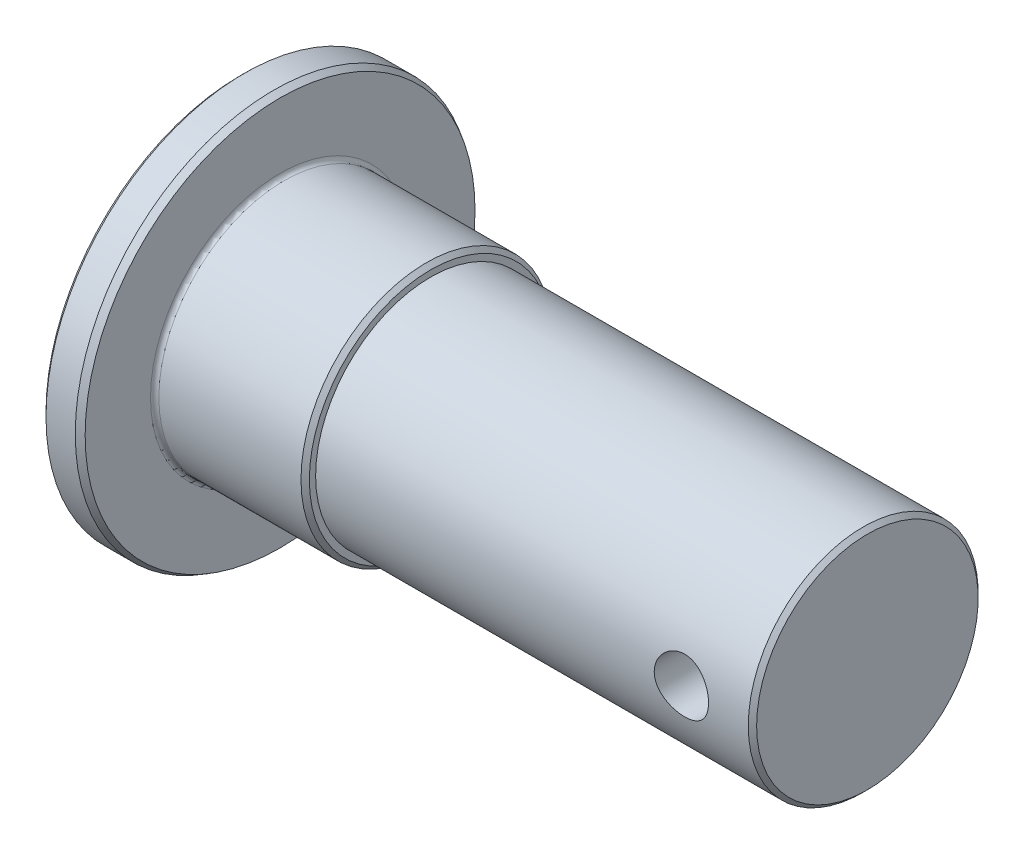
SolidWorks part; units mm, degrees
material "普通碳钢"
ref_plane "Front Plane" through (0, 0, 0) normal (0, 0, 1) x (1, 0, 0)
ref_plane "Top Plane" through (0, 0, 0) normal (0, 1, 0) x (1, 0, 0)
ref_plane "Right Plane" through (0, 0, 0) normal (1, 0, 0) x (0, 0, -1)
sketch "Sketch1" plane through (0, 0, 0) normal (0, 0, 1) x (1, 0, 0)
  line L0 (0, 0) -> (148.8633, 0) construction
  line L1 (0, 0) -> (0, 47.5)
  line L2 (0, -52.25) -> (0, 52.25) construction
  line L3 (0, 47.5) -> (8, 47.5)
  line L4 (9.5, 46.634) -> (9.5, 30)
  line L5 (9.5, 30) -> (45.5, 30)
  line L6 (45.5, 30) -> (45.5, 27.5)
  line L7 (45.5, 27.5) -> (150, 27.5)
  line L8 (150, 27.5) -> (150, 0)
  line L9 (45.5, -27.5) -> (150, -27.5) construction
  line L10 (45.5, -30) -> (45.5, -27.5) construction
  line L11 (9.5, -30) -> (45.5, -30) construction
  line L12 (9.5, -47.5) -> (9.5, -30) construction
  line L13 (0, -47.5) -> (9.5, -47.5) construction
  line L14 (0, 0) -> (150, 0)
  line L15 (8, 47.5) -> (9.5, 46.634)
  point P13 (150, 0)
  dimension "D1" = 55
  dimension "D2" = 104.5
  dimension "D3" = 36
  dimension "D4" = 95
  dimension "D5" = 60
  dimension "D6" = 150
  dimension "D7" = 1.5
  dimension "D8" = 30
revolve "Revolve1" add sketch "Sketch1" angle 360 about L14
fillet "Fillet1" radius 1 1 edges at (9.5, 0, 30)
chamfer "Chamfer1" distance 1 angle 45 3 edges at (0, 0, 47.5) (45.5, 0, 30) (150, 0, 27.5)
sketch "Sketch2" plane through (0, 0, 0) normal (0, 0, 1) x (1, 0, 0)
  line L0 (52.25, 0) -> (-52.25, 0) construction
  line L1 (150, -26.5) -> (150, 26.5) construction
  circle A0 centre (133, 0) radius 6.5
  dimension "D1" = 13
  dimension "D2" = 17
extrude "Cut-Extrude1" cut sketch "Sketch2" against normal through all and the other way through all
